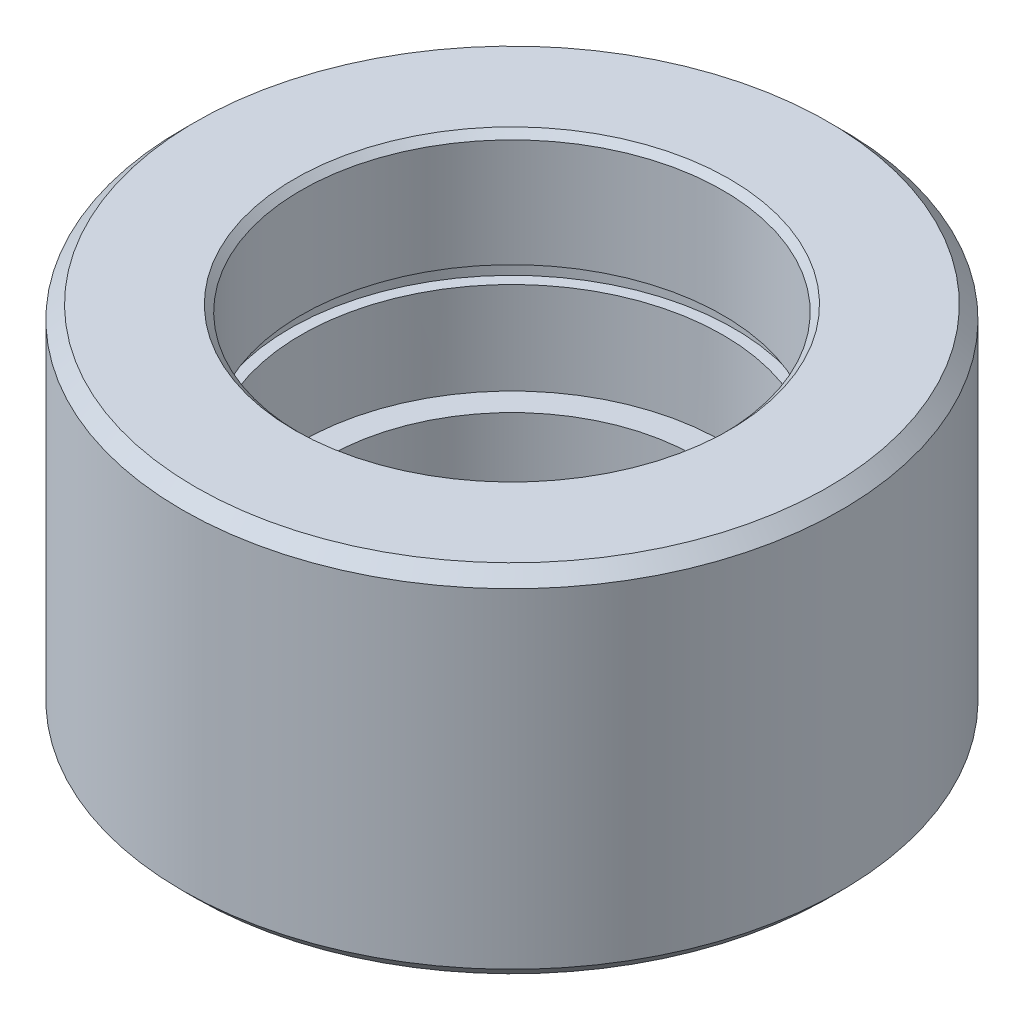
SolidWorks part; units mm, degrees
ref_plane "前视基准面" through (0, 0, 0) normal (0, 0, 1) x (1, 0, 0)
ref_plane "上视基准面" through (0, 0, 0) normal (0, 1, 0) x (1, 0, 0)
ref_plane "右视基准面" through (0, 0, 0) normal (1, 0, 0) x (0, 0, -1)
sketch "草图1" plane through (0, 0, 0) normal (0, 1, 0) x (1, 0, 0)
  circle A0 centre (0, 0) radius 25
  dimension "D1" = 50
extrude "凸台-拉伸1" add sketch "草图1" along normal blind 27
sketch "草图2" plane through (0, 27, 0) normal (0, 1, 0) x (1, 0, 0)
  circle A0 centre (0, 0) radius 16
  dimension "D1" = 32
extrude "切除-拉伸1" cut sketch "草图2" against normal blind 17
sketch "草图3" plane through (0, 10, 0) normal (0, 1, 0) x (1, 0, 0)
  circle A0 centre (0, 0) radius 14
  dimension "D1" = 28
extrude "切除-拉伸2" cut sketch "草图3" against normal through all
chamfer "倒角1" distance 1 angle 45 2 edges at (0, 0, 25) (0, 27, 25)
chamfer "倒角2" distance 0.5 angle 45 1 edges at (0, 27, 16)
sketch "草图4" plane through (0, 0, 0) normal (1, 0, 0) x (0, 0, -1)
  line L0 (16.5, 27) -> (-16.5, 27) construction
  line L1 (-16.85, 18.3) -> (-14.85, 18.3)
  line L2 (-16.85, 18.3) -> (-16.85, 17)
  line L3 (-16.85, 17) -> (-14.85, 17)
  line L4 (-14.85, 18.3) -> (-14.85, 17)
  line L5 (-16.85, 18.3) -> (-14.85, 17) construction
  line L6 (-16.85, 17) -> (-14.85, 18.3) construction
  point P0 (-15.85, 17.65)
  dimension "D1" = 16.85
  dimension "D2" = 1.3
  dimension "D3" = 8.7
  dimension "D4" = 2
revolve "切除-旋转1" cut sketch "草图4" angle 360 about axis through (0, 27, 0) along (0, -1, 0)
